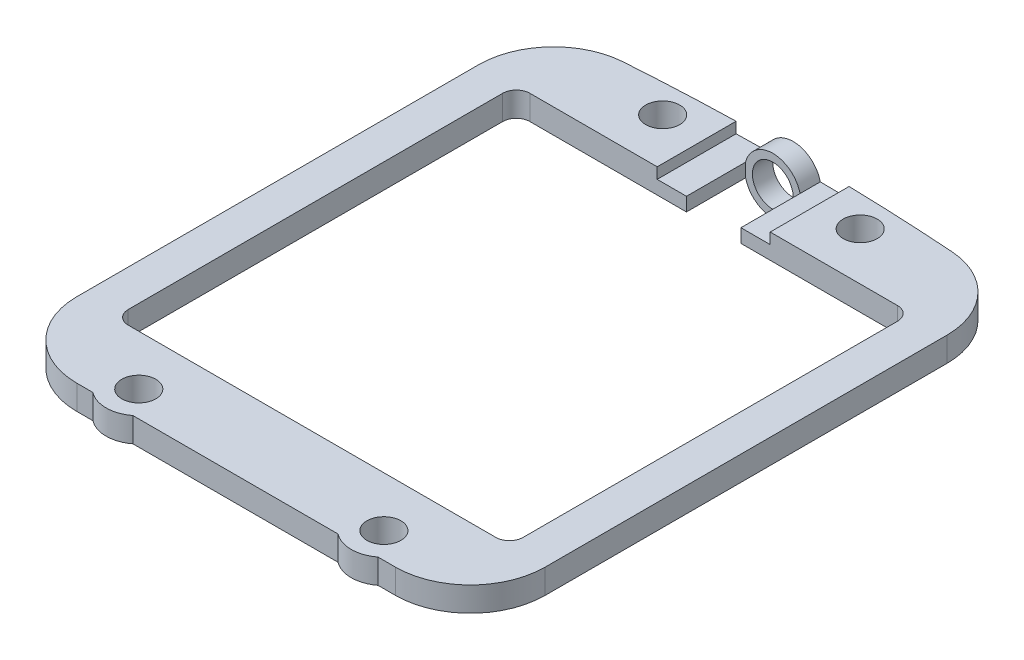
from build123d import *
from build123d.topology import SkipClean

# Parameters (mm, degrees)
BOSS_EXTRUDE_1_DEPTH      = 0.9
CUT_EXTRUDE_1_DEPTH       = 28.026205
CUT_EXTRUDE_1_DEPTH_BACK  = 28.026205
SKETCH_2_R                = 1.25
SKETCH_3_W                = 4
SKETCH_3_H                = 4.342956
CUT_EXTRUDE_2_DEPTH       = 1.8
SKETCH_4_W                = 8.3
SKETCH_4_H                = 6.175349
CUT_EXTRUDE3_DEPTH        = 0.8
BOSS_EXTRUDE_2_REACH      = 45.477
BOSS_EXTRUDE_2_END_RADIUS = 173.987356
SKETCH_10_R               = 2.061553
SKETCH_10_R_2             = 1.5
SKETCH_11_R               = 1.5
CUT_EXTRUDE_7_DEPTH       = 10


with BuildPart() as part:
    # Sketch 1 → Boss-Extrude 1 (new, symmetric)
    with BuildSketch(Plane(origin=(0, 0, 0), x_dir=(1, 0, 0), z_dir=(0, 1, 0))):
        with BuildLine():
            Line((-17.2, -14.827044), (-17.2, 14.686233))
            ThreePointArc((-17.2, 14.686233), (-15.721853, 18.437859), (-12.081928, 20.172956))
            ThreePointArc((-12.081928, 20.172956), (0, 20.592956), (12.081928, 20.172956))
            ThreePointArc((12.081928, 20.172956), (15.721853, 18.437859), (17.2, 14.686233))
            Line((17.2, 14.686233), (17.2, -14.827044))
            ThreePointArc((17.2, -14.827044), (15.589087, -18.716131), (11.7, -20.327044))
            Line((11.7, -20.327044), (10.41998, -20.327044))
            ThreePointArc((10.41998, -20.327044), (8.953692, -20.827044), (7.487405, -20.327044))
            Line((7.487405, -20.327044), (-7.583712, -20.327044))
            ThreePointArc((-7.583712, -20.327044), (-9.05, -20.827044), (-10.516288, -20.327044))
            Line((-10.516288, -20.327044), (-11.7, -20.327044))
            ThreePointArc((-11.7, -20.327044), (-15.589087, -18.716131), (-17.2, -14.827044))
        make_face()
        with BuildLine():
            Line((-13.5, -14.75), (13.5, -14.75))
            ThreePointArc((13.5, -14.75), (14.207107, -14.457107), (14.5, -13.75))
            Line((14.5, -13.75), (14.5, 13.75))
            ThreePointArc((14.5, 13.75), (14.207107, 14.457107), (13.5, 14.75))
            Line((13.5, 14.75), (-13.5, 14.75))
            ThreePointArc((-13.5, 14.75), (-14.207107, 14.457107), (-14.5, 13.75))
            Line((-14.5, 13.75), (-14.5, -13.75))
            ThreePointArc((-14.5, -13.75), (-14.207107, -14.457107), (-13.5, -14.75))
        make_face(mode=Mode.SUBTRACT)
    extrude(amount=BOSS_EXTRUDE_1_DEPTH, both=True)

    # Sketch 2 → Cut-Extrude 1 (cut, two sides: drawn at the far end of the back side and taken through both)
    with BuildSketch(Plane(origin=(0, 0, 0), x_dir=(1, 0, 0), z_dir=(0, 1, 0)).offset(-CUT_EXTRUDE_1_DEPTH_BACK)):
        with Locations(Location((-9.05, -18.427044, 0), (0, 0, 270))):
            Circle(SKETCH_2_R)
        with Locations(Location((8.953692, -18.427044, 0), (0, 0, 270))):
            Circle(SKETCH_2_R)
        with Locations(Location((-7.253142, 18.256885, 0), (0, 0, 270))):
            Circle(SKETCH_2_R)
        with Locations(Location((7.253142, 18.256885, 0), (0, 0, 270))):
            Circle(SKETCH_2_R)
    extrude(amount=CUT_EXTRUDE_1_DEPTH + CUT_EXTRUDE_1_DEPTH_BACK, mode=Mode.SUBTRACT)

    # Sketch 3 → Cut-Extrude 2 (cut)
    with BuildSketch(Plane(origin=(0, 0.9, 0), x_dir=(1, 0, 0), z_dir=(0, 1, 0))):
        with Locations((0, 16.921478)):
            Rectangle(SKETCH_3_W, SKETCH_3_H)
    extrude(amount=-CUT_EXTRUDE_2_DEPTH, mode=Mode.SUBTRACT)

    # Sketch 4 → Cut-Extrude3 (cut)
    with BuildSketch(Plane(origin=(0, 0.9, 0), x_dir=(1, 0, 0), z_dir=(0, 1, 0))):
        with Locations((0, 17.837674)):
            Rectangle(SKETCH_4_W, SKETCH_4_H)
    extrude(amount=-CUT_EXTRUDE3_DEPTH, mode=Mode.SUBTRACT)

    # Boss-Extrude 2: up to this cylinder (the profile starts inside it)
    boss_extrude_2_end = Plane(origin=(0, -0.4, 153.3944), z_dir=(0, -1, 0)) * Cylinder(BOSS_EXTRUDE_2_END_RADIUS, 439.928711, mode=Mode.PRIVATE)
    # Sketch 10 → Boss-Extrude 2 (add, up to the surface)
    with BuildSketch(Plane.XY.offset(-19.092956), mode=Mode.PRIVATE) as boss_extrude_2_sk1:
        with Locations((0, -0.4)):
            Circle(SKETCH_10_R)
        with Locations((0, -0.4)):
            Circle(SKETCH_10_R_2, mode=Mode.SUBTRACT)
    boss_extrude_2_tool1 = extrude(boss_extrude_2_sk1.sketch, amount=-BOSS_EXTRUDE_2_REACH, mode=Mode.PRIVATE) & boss_extrude_2_end
    add(boss_extrude_2_tool1.solids().sort_by_distance((-2.003243, -0.4, -19.092956))[0])

    # Sketch 11 → Cut-Extrude 7 (cut)
    with SkipClean():  # the faces are left unmerged after this step: merging them gives an invalid solid
        with BuildSketch(Plane.XY.offset(-19.092956)):
            with Locations((0, -0.4)):
                Circle(SKETCH_11_R)
        extrude(amount=-CUT_EXTRUDE_7_DEPTH, mode=Mode.SUBTRACT)


solid = part.part
